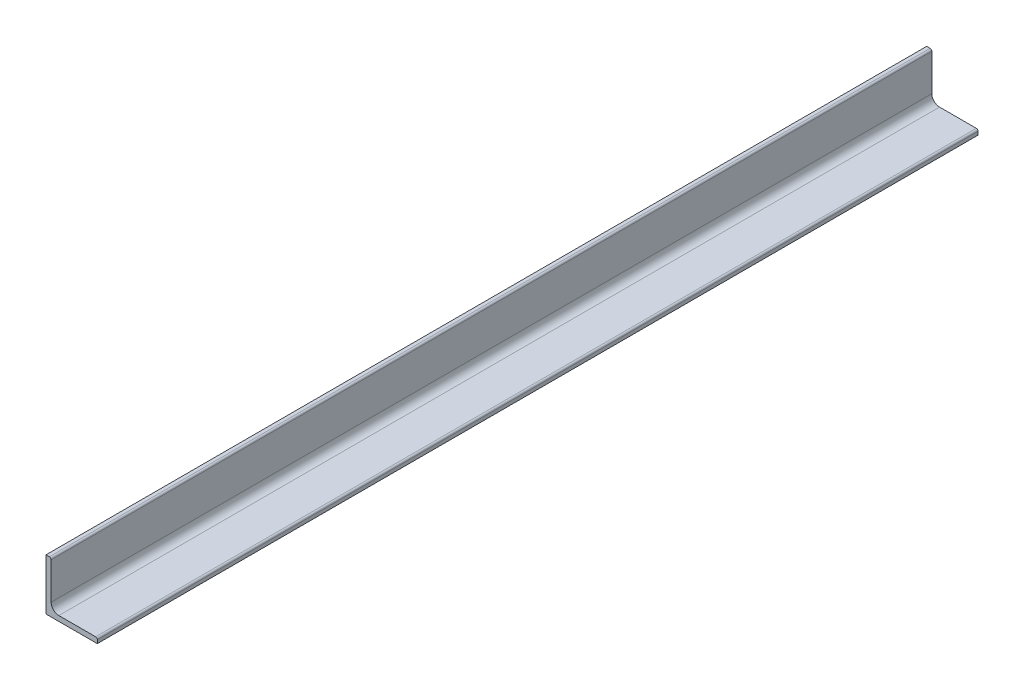
SolidWorks part; units mm, degrees
material "Plain Carbon Steel"
ref_plane "Plane1" through (0, 0, 0) normal (0, 0, 1) x (1, 0, 0)
ref_plane "Plane2" through (0, 0, 0) normal (0, 1, 0) x (1, 0, 0)
ref_plane "Plane3" through (0, 0, 0) normal (1, 0, 0) x (0, 0, -1)
sketch "Sketch1" plane through (0, 0, 0) normal (0, 0, 1) x (1, 0, 0)
  line L0 (0, 0) -> (0, 30)
  line L1 (0, 15) -> (3, 15) construction
  line L2 (3, 29) -> (3, 7.5)
  line L3 (7.5, 3) -> (29, 3)
  line L4 (15, 3) -> (15, 0) construction
  line L5 (30, 0) -> (0, 0)
  line L6 (0, 30) -> (2, 30)
  line L7 (30, 0) -> (30, 2)
  arc A0 (30, 2) -> (29, 3) centre (29, 2) ccw
  arc A1 (2, 30) -> (3, 29) centre (2, 29) cw
  arc A2 (7.5, 3) -> (3, 7.5) centre (7.5, 7.5) cw
  point P10 (15, 0)
  point P14 (0, 15)
  point P15 (3, 15)
  point P16 (15, 3)
  point P17 (3, 30)
  point P18 (30, 3)
  point P21 (30, 3)
  point P24 (3, 30)
extrude "Boss-Extrude1" add sketch "Sketch1" along normal mid plane 515 contours L2 A2 L3 A0 L7 L5 L0 L6 A1
equation "\"D2@Sketch1\" = \"D1@Sketch1\" / 3"
